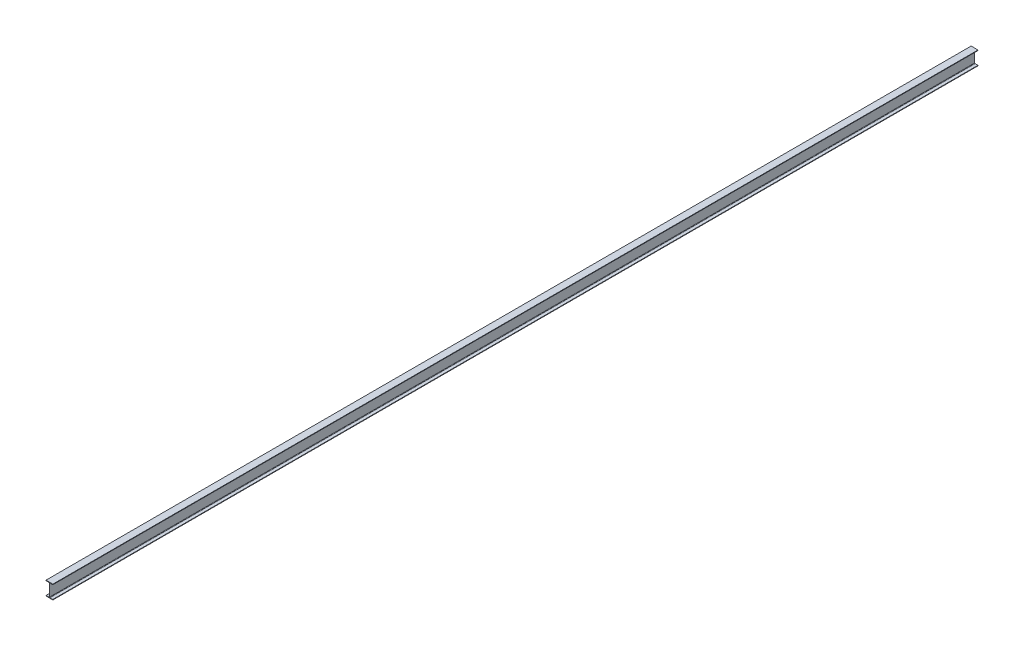
from build123d import *

# Parameters (mm, degrees)
BOSS_EXTRUDE1_DEPTH = 16840


with BuildPart() as part:
    # Sketch1 → Boss-Extrude1 (new body)
    with BuildSketch(Plane.XY):
        with BuildLine():
            Line((62.5, 0), (-62.5, 0))
            Line((-62.5, 0), (-62.5, 9))
            Line((-62.5, 9), (-11, 9))
            ThreePointArc((-11, 9), (-5.343145751, 11.343145751), (-3, 17))
            Line((-3, 17), (-3, 233))
            ThreePointArc((-3, 233), (-5.343145751, 238.656854249), (-11, 241))
            Line((-11, 241), (-62.5, 241))
            Line((-62.5, 241), (-62.5, 250))
            Line((-62.5, 250), (62.5, 250))
            Line((62.5, 250), (62.5, 241))
            Line((62.5, 241), (11, 241))
            ThreePointArc((11, 241), (5.343145751, 238.656854249), (3, 233))
            Line((3, 233), (3, 17))
            ThreePointArc((3, 17), (5.343145751, 11.343145751), (11, 9))
            Line((11, 9), (62.5, 9))
            Line((62.5, 9), (62.5, 0))
        make_face()
    extrude(amount=BOSS_EXTRUDE1_DEPTH)


solid = part.part
